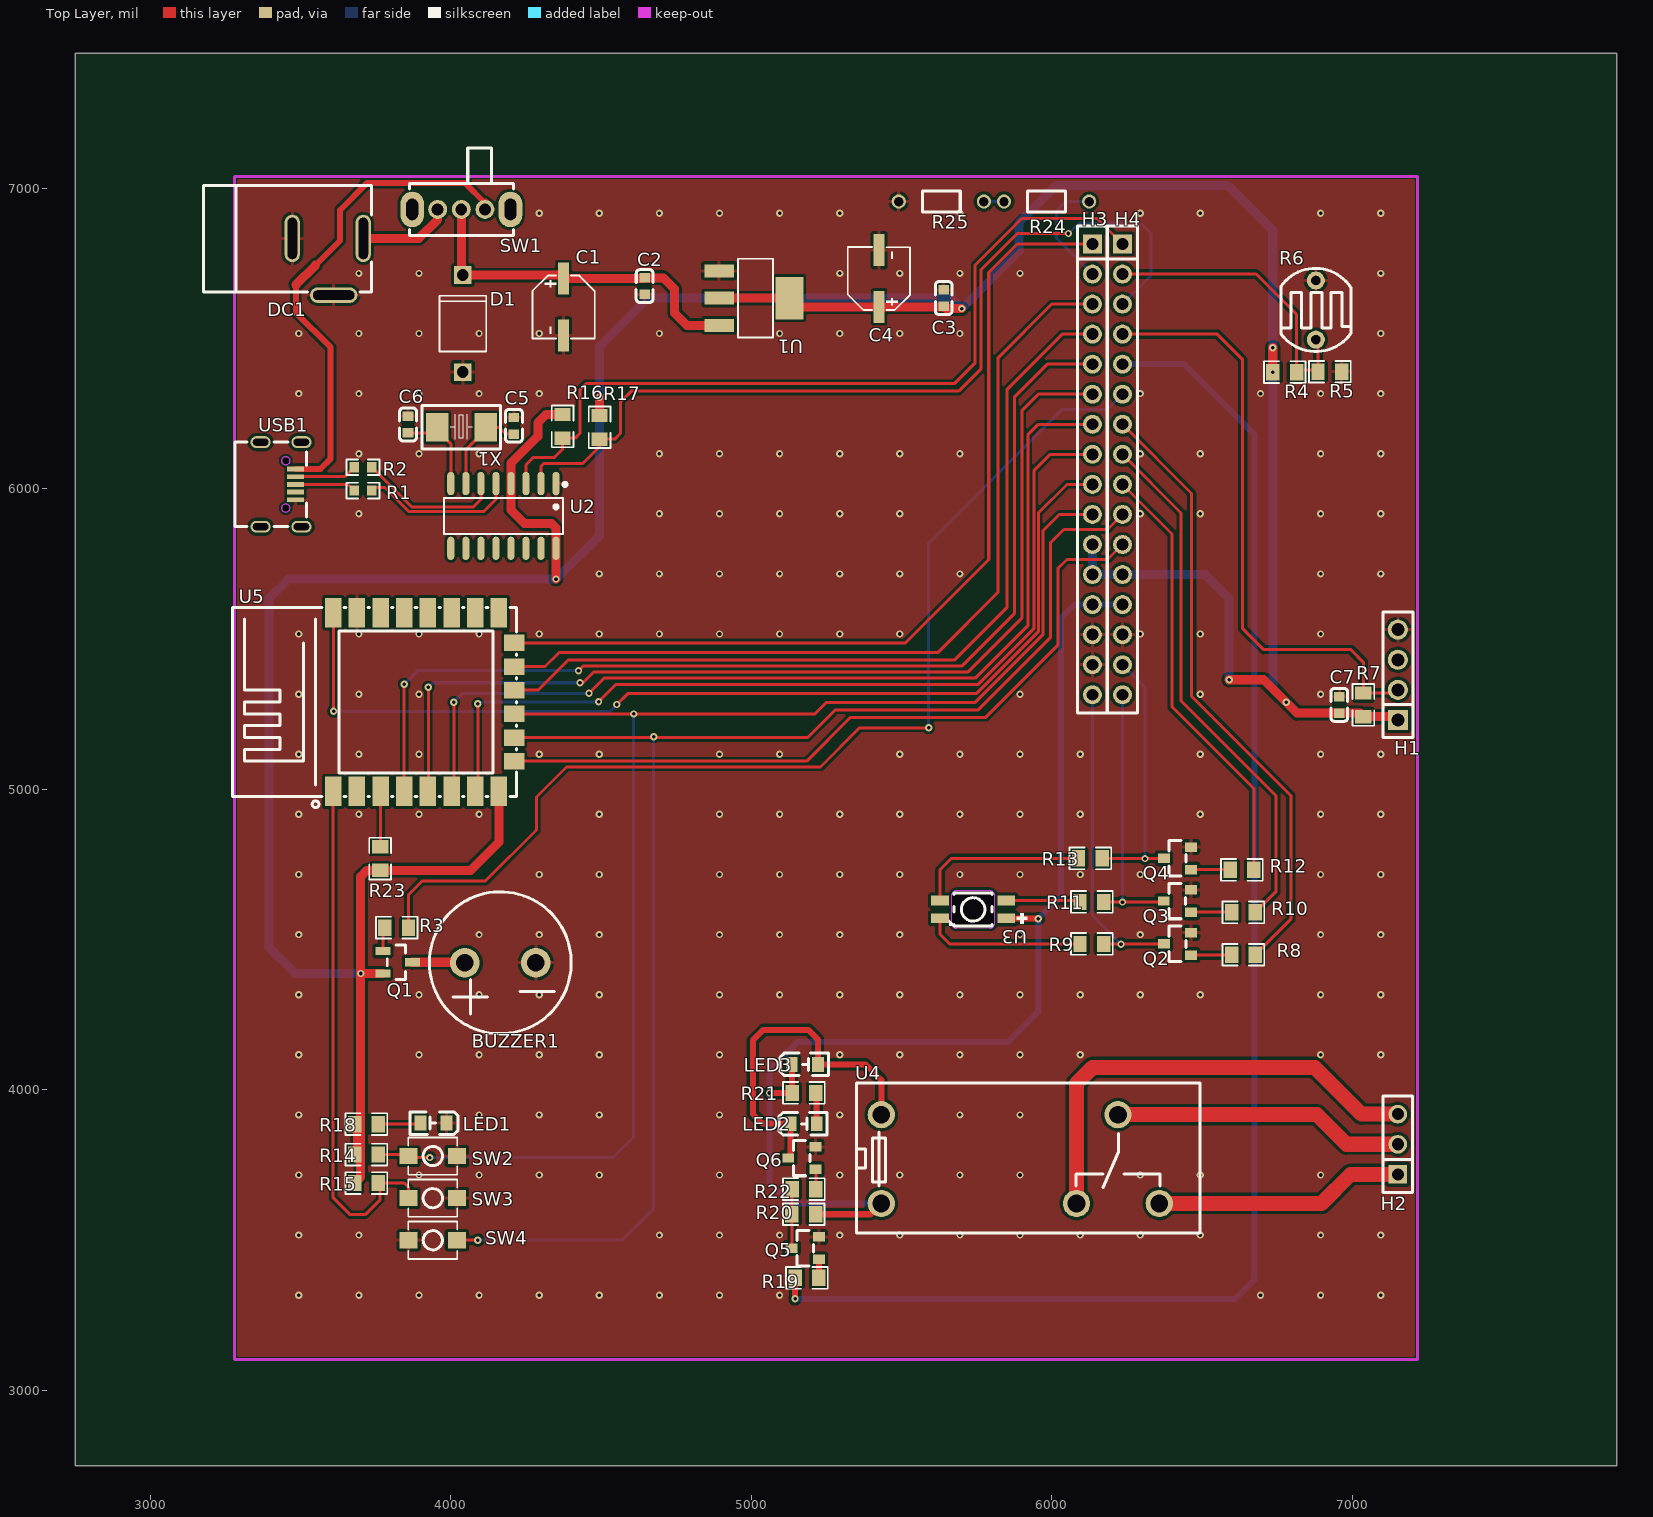
[diagram p0: Top Layer view]
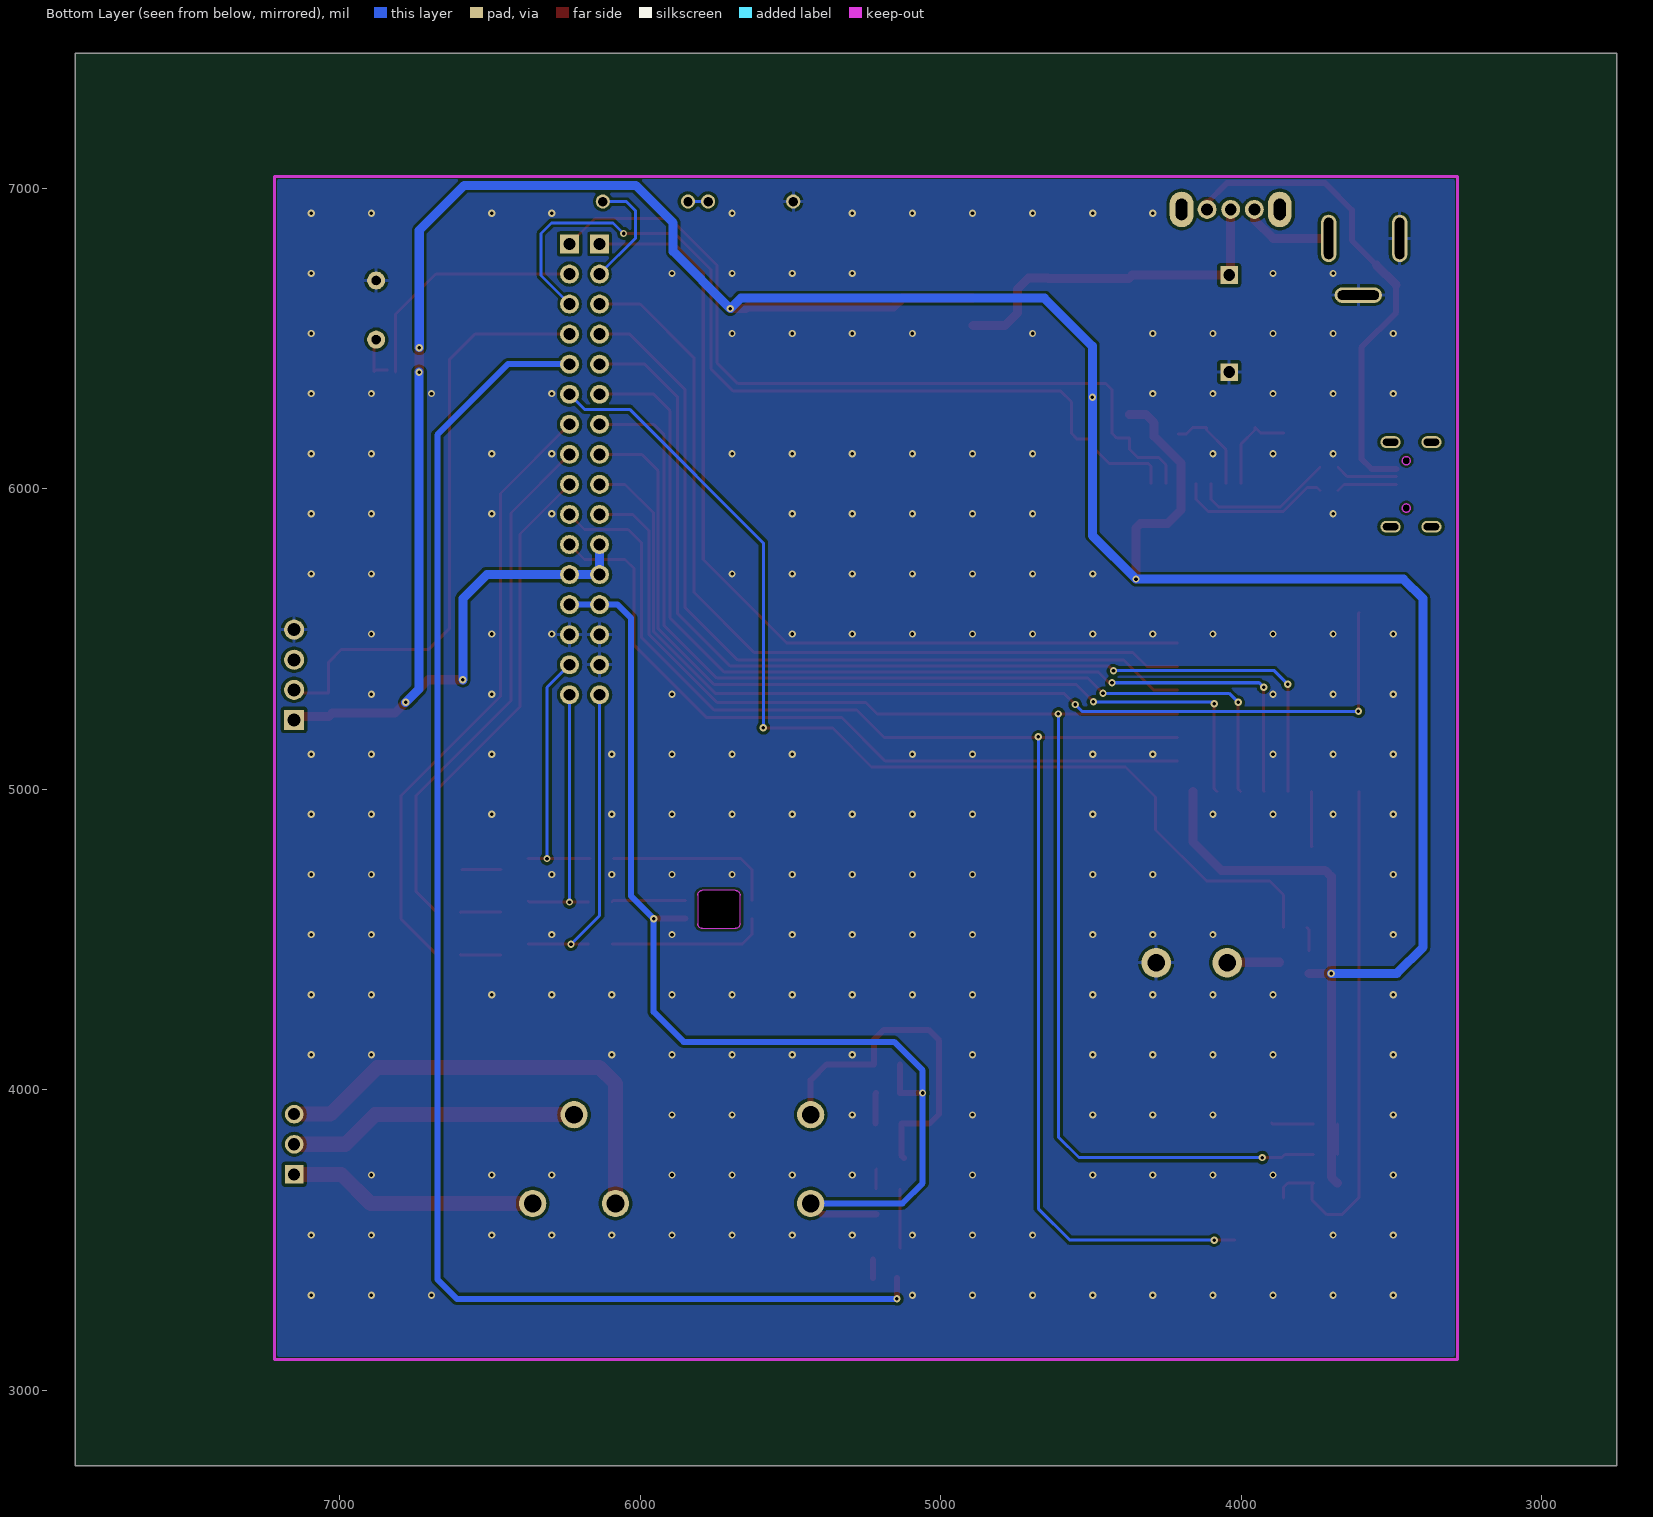
[diagram p1: Bottom Layer view, seen from below]
# Altium PCB MISC51905.pcbdoc
Units mil, origin at the board's own origin, x right, y up, seen from the top; angles counter-clockwise.
Board outline 5130 x 4700 mil, 2 copper layers (Top Layer, Bottom Layer), stack 62.206 mil thick; 59 components, 57 nets, 207 pads, 250 vias.

## Layer stack, top to bottom
Top Solder Mask Layer: solder mask 0.394, Dk 3.3
Top Layer: signal copper 1.379
Dielectric1: surface 59.449, FR4, Dk 4.5
Bottom Layer: signal copper 1.378
Bottom Solder Mask Layer: solder mask 0.394, Dk 3.3

## Board outline
7880,2750 2750,2750 2750,7450 7880,7450

## Design rules (kind name [scope] priority, off if disabled: settings)
BoardOutlineClearance copperThickness2oz_1 [All] p2 off: genericclearance=7.99 ignorepadtopadclearanceinfootprint=FALSE except(0: Arc-SplitContinuation Track-SplitContinuation SMDPad-SplitContinuation THPad-SplitContinuation Via-SplitContinuation Fill-SplitContinuation Region-SplitContinuation Poly-SplitContinuation Text-SplitContinuation Hole-SplitContinuation; 5.98: Arc-CutoutEdge SMDPad-CutoutEdge THPad-CutoutEdge Via-CutoutEdge Fill-CutoutEdge Region-CutoutEdge Text-CutoutEdge; 6.93: Hole-OutlineEdge Hole-CutoutEdge; 10: Poly-OutlineEdge Poly-CutoutEdge; 11.81: Arc-OutlineEdge Track-OutlineEdge SMDPad-OutlineEdge THPad-OutlineEdge Via-OutlineEdge Fill-OutlineEdge Region-OutlineEdge Text-OutlineEdge Track-CutoutEdge)
BoardOutlineClearance copperThickness1oz_1 [All] p4: genericclearance=4.02 ignorepadtopadclearanceinfootprint=FALSE except(0: Arc-SplitContinuation Track-SplitContinuation SMDPad-SplitContinuation THPad-SplitContinuation Via-SplitContinuation Fill-SplitContinuation Region-SplitContinuation Poly-SplitContinuation Text-SplitContinuation Hole-SplitContinuation; 6: SMDPad-CutoutEdge THPad-CutoutEdge Via-CutoutEdge Fill-CutoutEdge Region-CutoutEdge Text-CutoutEdge; 6.93: Hole-OutlineEdge Hole-CutoutEdge; 10: Poly-OutlineEdge Poly-CutoutEdge; 11.8: Arc-OutlineEdge Track-OutlineEdge SMDPad-OutlineEdge THPad-OutlineEdge Via-OutlineEdge Fill-OutlineEdge Region-OutlineEdge Text-OutlineEdge; 11.81: Arc-CutoutEdge Track-CutoutEdge)
Clearance copperThickness2oz [All] p1 off: gap=7.99 ignorepadtopadclearanceinfootprint=FALSE except(5.98: SMDPad-Track SMDPad-SMDPad THPad-Track SMDPad-THPad THPad-THPad Track-Via SMDPad-Via THPad-Via Via-Via Fill-Track Region-Track Fill-SMDPad Region-SMDPad Fill-THPad Region-THPad Fill-Via Region-Via Fill-Fill Fill-Region Region-Region Arc-Track Arc-SMDPad Arc-THPad Arc-Via Fill-Arc Region-Arc Arc-Arc Text-Track SMDPad-Text Text-THPad Text-Via Fill-Text Region-Text Arc-Text Text-Text; 6.93: Hole-Track Hole-SMDPad Hole-THPad Hole-Via Fill-Hole Region-Hole Hole-Arc Hole-Text; 10: Poly-Track Poly-SMDPad Poly-THPad Poly-Via Poly-Fill Poly-Region Poly-Poly Poly-Arc Poly-Text Poly-Hole)
Clearance copperThickness1oz [All] p3: gap=4.02 ignorepadtopadclearanceinfootprint=FALSE except(5.98: SMDPad-Track SMDPad-SMDPad THPad-Track SMDPad-THPad THPad-THPad Track-Via SMDPad-Via THPad-Via Via-Via Fill-Track Region-Track Fill-SMDPad Region-SMDPad Fill-THPad Region-THPad Fill-Via Region-Via Fill-Fill Fill-Region Region-Region; 6: Arc-Track Arc-SMDPad Arc-THPad Arc-Via Fill-Arc Region-Arc Arc-Arc Text-Track SMDPad-Text Text-THPad Text-Via Fill-Text Region-Text Arc-Text Text-Text; 6.93: Hole-Track Hole-SMDPad Hole-THPad Hole-Via Fill-Hole Region-Hole Hole-Arc Hole-Text; 10: Poly-Track Poly-SMDPad Poly-THPad Poly-Via Poly-Fill Poly-Region Poly-Poly Poly-Arc Poly-Text Poly-Hole)
DiffPairsRouting differentialPair [All] p1: maxlimit=6 minlimit=6 mostfreqgap=6 toplayer_minwidth=5 toplayer_prefwidth=10 toplayer_maxwidth=100 toplayer_mingap=6 toplayer_prefgap=6 toplayer_maxgap=6 bottomlayer_minwidth=5 bottomlayer_prefwidth=10 bottomlayer_maxwidth=100 bottomlayer_mingap=6 bottomlayer_prefgap=6 bottomlayer_maxgap=6 maxuncoupledlength=10
HoleToHoleClearance otherClearance [All] p1: gap=11.81 allowstackedmicrovias=TRUE
Length netLength [All] p1: minlimit=0 maxlimit=0
MatchedLengths netLengthTolerance [All] p1: tolerance=1000
PasteMaskExpansion pasteMaskExpansion [All] p1: expansion=0
PlaneConnect innerPlane [All] p1: planeconnectstyle=Relief reliefexpansion=20 reliefentries=4 reliefconductorwidth=10 reliefairgap=10
PolygonConnect copperRegion [(InNet('GND'))] p1: connectstyle=Relief reliefconductorwidth=10 reliefentries=4 polygonreliefangle="90 Angle" airgapwidth=10 via.connectstyle=Relief via.reliefconductorwidth=10 via.reliefentries=4 via.polygonreliefangle="90 Angle" via.airgapwidth=10
RoutingVias viaSize [All] p1: holewidth=12.01 width=24.02 viastyle="Through Hole" minholewidth=11.81 minwidth=19.68 maxholewidth=248.03 maxwidth=393.7
SolderMaskExpansion solderMaskExpansion [IsVia] p1: expansion=-1000 istentingtop=TRUE
SolderMaskExpansion solderMaskExpansion [All] p2: expansion=2 istentingtop=FALSE
Width copperThickness2oz_2 [All] p1 off: maxlimit=100 minlimit=8 preferedwidth=10
Width copperThickness1oz_2 [All] p2: maxlimit=100 minlimit=5 preferedwidth=10

## Components (designator, comment, footprint, x,y, rotation, side; value= is the part's Value field where it differs from the comment)
BUZZER1 "buzzer" BUZ-TH_BD12.0-P6.00-D0.9-RD 4164.88,4423.36 r180 top
C1 "10uF" C_Ele_SMD_5x5.4mm 4375,6605 r270 top
C2 "100nF" C0603 4645,6675 r90 top
C3 "100nF" C0603 5640,6635 r270 top
C4 "10uF" C_Ele_SMD_5x5.4mm 5425,6700 r90 top
C5 "22pF" C0603 4210,6210 r270 top
C6 "22pF" C0603 3857.75,6214.29 r270 top
C7 "100nF" C0603 6956.48,5281.48 r270 top
D1 "SMA_DIODE" SOD-57_BD3.8-L4.6-P9.00-D0.8-RD 4040,6550 r270 top
DC1 "" DC-2.0 3585.7,6844.2 r180 top
H1 "" HDR-TH_4P-P2.54-V-F 7151.48,5381.48 r90 top
H2 "" HDR-TH_3P-P2.54-V-F 7151.08,3819.36 r90 top
H3 "" HDR-TH_16P-P2.54-V-F 6135,6065 r270 top
H4 "" HDR-TH_16P-P2.54-V-F 6235,6065 r270 top
LED1 "" LED_0805 3940,3890 r180 top
LED2 "" LED_0805 5176.09,3887.47 r0 top
LED3 "" LED_0805 5180,4085 r0 top
Q1 "" S8550P_SOT 3825,4425 r180 top
Q2 "" S8050_SOT-23 6418.13,4485.78 r0 top
Q3 "" S8050_SOT-23 6417.7,4628.77 r0 top
Q4 "" S8050_SOT-23 6418.13,4770.78 r0 top
Q5 "" S8050_SOT-23 5179.42,3473.63 r0 top
Q6 "" S8050_SOT-23 5168.07,3773.63 r0 top
R1 "27R" R0603 3707.89,5994.43 r180 top
R2 "27R" R0603 3707.89,6072.13 r180 top
R3 "1K" R0805 3820,4540 r180 top
R4 "10K" R0805 6774.9,6388.36 r0 top
R5 "4.7K" R0805 6925,6390 r0 top
R6 "GL7528" RES-TH_L7.0-W5.9-P5.00-D0.5 6878.39,6595.1 r0 top
R7 "4.7K" R0805 7036.48,5281.48 r270 top
R8 "1.5K" R0805 6637.43,4450.05 r180 top
R9 "1K" R0805 6133.13,4485.78 r180 top
R10 "1.5K" R0805 6637.43,4591.12 r180 top
R11 "1K" R0805 6133.13,4625.78 r180 top
R12 "1.5K" R0805 6632.43,4732.47 r180 top
R13 "1K" R0805 6128.13,4770.78 r180 top
R14 "10K" R0805 3719.38,3785 r0 top
R15 "10K" R0805 3719.38,3690.3 r0 top
R16 "10K" R0805 4371.73,6208.26 r270 top
R17 "10K" R0805 4495,6205 r270 top
R18 "4.7K" R0805 3719.38,3886.21 r0 top
R19 "1.5K" R0805 5185,3375 r0 top
R20 "1.5K" R0805 5174.42,3586.47 r0 top
R21 "10K" R0805 5175,3990 r180 top
R22 "1.5K" R0805 5175,3670 r0 top
R23 "10K" R0805 3765,4770 r90 top
R24 "10K" Res_1/8W 5982.44,6953.68 r0 top
R25 "4.7K" Res_1/8W 5632.16,6953.68 r0 top
SW1 "" 拨动开关_侧 4035,6930 r180 top
SW2 "" Key_SMD_3x4x2 3940,3780 r0 top
SW3 "" Key_SMD_3x4x2 3940,3640 r0 top
SW4 "" Key_SMD_3x4x2 3940,3500 r180 top
U1 "AMS1117-3.3" SOT-223-3_L6.5-W3.4-P2.30-LS7.0-BR 5010,6635 r180 top
U2 "CH340G" SOIC-16_L9.9-W3.9-P1.27-LS6.0-BL 4175,5910 r180 top
U3 "6028-ZRGBF-SMD-H2" LED-SMD_4P-L3.2-W2.8_ZRGBF-SMD-H2 5738.13,4600.78 r180 top
U4 "SSKD6132" RELAY-TH_G2R-1 5895,3770 r0 top
U5 "ESP8266" WIFIM-SMD_ESP-12F-ESP8266MOD 3909.99,5290.81 r0 top
USB1 "" USB_Micro 3435,6015 r270 top
X1 "CRYSTAL" CRYSTAL-SMD_L5.0-W3.2 4035,6205 r180 top

## Footprints (in the part's own frame and the unit in brackets; to place one, negate y for a bottom-side part, rotate by r counter-clockwise, add the part's x,y. Pads: shape width x height; smd on the part's side, far side on the other; paste and mask are expansions set on the pad)
BUZ-TH_BD12.0-P6.00-D0.9-RD [mm]
  round 2.5 hole 1.5 paste+0 mask+0.05: 1(-3,0) 2(3,0)
  silkscreen extent -5.99,-5.99 5.99,5.99
C0603 [mm]
  rect 0.8x0.9 smd: 1(-0.7,0) 2(0.7,0)
  silkscreen extent -1.39,-0.71 1.39,0.71
C_Ele_SMD_5x5.4mm [mm]
  rect 2.7x0.91 smd paste+0 mask+0.051: 1(-2.4,0) 2(2.4,0)
  silkscreen extent -2.66,-2.62 2.66,2.65
CRYSTAL-SMD_L5.0-W3.2 [mm]
  rect 1.9x2.4 smd: 1(-2.05,0) 2(2.05,0)
  silkscreen extent -3.32,-1.85 3.33,1.85
DC-2.0 [mil]
  oval 157.5x51.2 hole 31.5 slot 137.8 at 0 deg paste+0 mask+2: 2(-24.7,199.5)
  oval 51.2x157.5 hole 31.5 slot 137.8 at 90 deg paste+0 mask+2: 3(113.1,10.5) 4(-123.1,10.5)
  silkscreen extent -151,-165 408,190
HDR-TH_3P-P2.54-V-F [mil]
  rect 62x62 hole 40.16: 1(-100,0)
  round 62 hole 40.16: 2(0,0) 3(100,0)
  silkscreen extent -160,-49 160,49
HDR-TH_4P-P2.54-V-F [mm]
  rect 1.7x1.7 hole 1.1: 1(-3.81,0)
  round 1.7 hole 1.1: 2(-1.27,0) 3(1.27,0) 4(3.81,0)
  silkscreen extent -5.29,-1.27 5.29,1.27
HDR-TH_16P-P2.54-V-F [mm]
  rect 1.6x1.6 hole 1: 1(-19.05,0)
  round 1.6 hole 1: 2(-16.51,0) 3(-13.97,0) 4(-11.43,0) 5(-8.89,0) 6(-6.35,0) 7(-3.81,0) 8(-1.27,0) 9(1.27,0) 10(3.81,0) 11(6.35,0) 12(8.89,0) 13(11.43,0) 14(13.97,0) 15(16.51,0) 16(19.05,0)
  silkscreen extent -20.57,-1.25 20.57,1.25
Key_SMD_3x4x2 [mm]
  rect 1.53x1.36 smd paste+0 mask+0.051: 1(-2.035,0) 2(2.035,0)
  silkscreen extent -2.08,-1.58 2.08,1.58
LED-SMD_4P-L3.2-W2.8_ZRGBF-SMD-H2 [mm]
  rect 1.5x0.82 smd: 1(2.8,0.75) 2(-2.8,0.75) 3(2.8,-0.75) 4(-2.8,-0.75)
  Board Outline Layer lines w0.003: 1.8,1.2 ccw(c1.4,1.2) 1.4,1.6 -1.4,1.6 ccw(c-1.4,1.2) -1.8,1.2 -1.8,-1.2 ccw(c-1.4,-1.2) -1.406,-1.6 ccw(c-1.413,-1.2) -1.4,-1.6 1.4,-1.6 ccw(c1.4,-1.2) 1.8,-1.2 1.8,1.2
  Board Outline Layer region: 1.8,-1.2 1.79,-1.289 1.76,-1.374 1.713,-1.45 1.649,-1.513 1.574,-1.561 1.489,-1.59 1.4,-1.6 1.4,-1.6 -1.4,-1.6 -1.403,-1.6 -1.406,-1.6 -1.494,-1.589 -1.578,-1.559 -1.652,-1.511 -1.714,-1.448 -1.761,-1.372 -1.79,-1.288 -1.8,-1.2 -1.8,-1.2 -1.8,-1.2 -1.8,1.2 -1.79,1.289 -1.76,1.374 -1.713,1.449 -1.649,1.513 -1.574,1.56 -1.489,1.59 -1.4,1.6 1.4,1.6 1.4,1.6 1.489,1.59 1.574,1.561 1.649,1.513 1.713,1.45 1.76,1.374 1.79,1.289 1.8,1.2 1.8,-1.2
  Board Outline Layer region: 1.8,-1.2 1.79,-1.289 1.76,-1.374 1.713,-1.45 1.649,-1.513 1.574,-1.561 1.489,-1.59 1.4,-1.6 1.4,-1.6 -1.4,-1.6 -1.403,-1.6 -1.406,-1.6 -1.494,-1.589 -1.578,-1.559 -1.652,-1.511 -1.714,-1.448 -1.761,-1.372 -1.79,-1.288 -1.8,-1.2 -1.8,-1.2 -1.8,-1.2 -1.8,1.2 -1.79,1.289 -1.76,1.374 -1.713,1.449 -1.649,1.513 -1.574,1.56 -1.489,1.59 -1.4,1.6 1.4,1.6 1.4,1.6 1.489,1.59 1.574,1.561 1.649,1.513 1.713,1.45 1.76,1.374 1.79,1.289 1.8,1.2 1.8,-1.2
  Multi-Layer board cut-out: 1.8,-1.2 1.79,-1.289 1.76,-1.374 1.713,-1.45 1.649,-1.513 1.574,-1.561 1.489,-1.59 1.4,-1.6 1.4,-1.6 -1.4,-1.6 -1.403,-1.6 -1.406,-1.6 -1.494,-1.589 -1.578,-1.559 -1.652,-1.511 -1.714,-1.448 -1.761,-1.372 -1.79,-1.288 -1.8,-1.2 -1.8,-1.2 -1.8,-1.2 -1.8,1.2 -1.79,1.289 -1.76,1.374 -1.713,1.449 -1.649,1.513 -1.574,1.56 -1.489,1.59 -1.4,1.6 1.4,1.6 1.4,1.6 1.489,1.59 1.574,1.561 1.649,1.513 1.713,1.45 1.76,1.374 1.79,1.289 1.8,1.2 1.8,-1.2
  silkscreen extent -4.57,-1.4 2.03,1.4
LED_0805 [mm]
  rect 1x1.25 smd paste+0 mask+0.051: 1(-1.15,0.005) 2(1.05,0.005)
  silkscreen extent -2.15,-0.94 1.93,0.97
R0603 [mil]
  rect 31.75x34.02 smd paste-3937.01 mask+2: 1(-29.66,0) 2(29.66,0)
  silkscreen extent -55,-26 55,26
R0805 [mm]
  rect 1.133x1.377 smd paste-100 mask+0.051: 1(-1,0) 2(1,0)
  silkscreen extent -1.76,-0.92 1.76,0.92
RELAY-TH_G2R-1 [mm]
  round 2.3 hole 1.5: 1(-11.75,-3.75) 2(4.75,-3.75) 3(11.75,-3.75) 4(8.25,3.75) 5(-11.75,3.75)
  silkscreen extent -13.83,-6.26 15.17,6.44
RES-TH_L7.0-W5.9-P5.00-D0.5 [mil]
  round 60 hole 30 slot 30.2 at 90 deg: 1(0,-98.42) 2(0,98.43)
  silkscreen extent -116,-138 116,139
Res_1/8W [mil]
  round 47.2 hole 31.5 paste+0 mask+2: 1(-141.7,2.48) 2(141.7,2.48)
  silkscreen extent -63,-33 63,38
S8050_SOT-23 [mm]
  rect 1x0.8 smd paste+0 mask+0.051: 1(1.15,-0.95) 2(1.15,0.95) 3(-1.15,0)
  silkscreen extent -0.7,-1.5 0.7,1.5
S8550P_SOT [mil]
  rect 49.2x27.6 smd paste+0 mask+2: 1(50.84,-37.4) 2(50.84,37.4) 3(-47.56,0)
  silkscreen extent -24,-58 37,58
SOD-57_BD3.8-L4.6-P9.00-D0.8-RD [mm]
  rect 1.5x1.5 hole 1: 1(-4.1,0) 2(4.1,0)
  silkscreen extent -2.36,-1.98 2.36,1.98
SOIC-16_L9.9-W3.9-P1.27-LS6.0-BL [mil]
  oval 23.7x77.6 smd: 1(-175,-107.7) 2(-125,-107.7) 3(-75,-107.7) 4(-25,-107.7) 5(25,-107.7) 6(75,-107.7) 7(125,-107.7) 8(175,-107.7) 9(175,107.7) 10(125,107.7) 11(75,107.7) 12(25,107.7) 13(-25,107.7) 14(-75,107.7) 15(-125,107.7) 16(-175,107.7)
  silkscreen extent -211,-111 198,60
SOT-223-3_L6.5-W3.4-P2.30-LS7.0-BR [mm]
  rect 2.5x1.1 smd: 1(2.97,-2.3) 2(2.97,0) 3(2.97,2.3)
  rect 2.34x3.6 smd: 4(-2.97,0)
  silkscreen extent -1.57,-3.33 1.37,3.33
USB_Micro [mm]
  rect 0.4x1.4 smd paste-100 mask+0.05: 1(-1.3,1.225) 2(-0.65,1.225) 3(0,1.225) 4(0.65,1.225) 5(1.3,1.225)
  oval 1x1.7 hole 0.6 slot 1.3 at 90 deg paste+0 mask+0.05: 6(-3.575,-1.725) 6(-3.575,1.725) 6(3.575,-1.725) 6(3.575,1.725)
  Board Outline Layer circle w0.003: c-2,0.4 r0.35
  Board Outline Layer circle w0.003: c2,0.4 r0.35
  Board Outline Layer region: -2,0.75 -1.848,0.715 -1.726,0.618 -1.659,0.478 -1.659,0.322 -1.726,0.182 -1.848,0.085 -2,0.05 -2,0.05 -2.152,0.085 -2.274,0.182 -2.341,0.322 -2.341,0.478 -2.274,0.618 -2.152,0.715 -2,0.75
  Board Outline Layer region: -2,0.75 -1.922,0.741 -1.848,0.715 -1.782,0.674 -1.726,0.618 -1.685,0.552 -1.659,0.478 -1.65,0.4 -1.659,0.322 -1.685,0.248 -1.726,0.182 -1.782,0.126 -1.848,0.085 -1.922,0.059 -2,0.05 -2.078,0.059 -2.152,0.085 -2.218,0.126 -2.274,0.182 -2.315,0.248 -2.341,0.322 -2.35,0.4 -2.341,0.478 -2.315,0.552 -2.274,0.618 -2.218,0.674 -2.152,0.715 -2.078,0.741
  Board Outline Layer region: 2,0.75 2.152,0.715 2.274,0.618 2.341,0.478 2.341,0.322 2.274,0.182 2.152,0.085 2,0.05 2,0.05 1.848,0.085 1.726,0.182 1.659,0.322 1.659,0.478 1.726,0.618 1.848,0.715 2,0.75
  Board Outline Layer region: 2,0.75 2.078,0.741 2.152,0.715 2.218,0.674 2.274,0.618 2.315,0.552 2.341,0.478 2.35,0.4 2.341,0.322 2.315,0.248 2.274,0.182 2.218,0.126 2.152,0.085 2.078,0.059 2,0.05 1.922,0.059 1.848,0.085 1.782,0.126 1.726,0.182 1.685,0.248 1.659,0.322 1.65,0.4 1.659,0.478 1.685,0.552 1.726,0.618 1.782,0.674 1.848,0.715 1.922,0.741
  Multi-Layer board cut-out: -2,0.75 -1.848,0.715 -1.726,0.618 -1.659,0.478 -1.659,0.322 -1.726,0.182 -1.848,0.085 -2,0.05 -2,0.05 -2.152,0.085 -2.274,0.182 -2.341,0.322 -2.341,0.478 -2.274,0.618 -2.152,0.715 -2,0.75
  Multi-Layer board cut-out: 2,0.75 2.152,0.715 2.274,0.618 2.341,0.478 2.341,0.322 2.274,0.182 2.152,0.085 2,0.05 2,0.05 1.848,0.085 1.726,0.182 1.659,0.322 1.659,0.478 1.726,0.618 1.848,0.715 2,0.75
  silkscreen extent -3.57,-3.87 3.57,2.14
WIFIM-SMD_ESP-12F-ESP8266MOD [mm]
  rect 1.4x2.5 smd: 1(-7.651,-7.551) 2(-5.651,-7.551) 3(-3.651,-7.551) 4(-1.651,-7.551) 5(0.349,-7.551) 6(2.349,-7.551) 7(4.349,-7.551) 8(6.349,-7.551) 9(6.349,7.549) 10(4.349,7.55) 11(2.349,7.551) 12(0.349,7.551) 13(-1.651,7.55) 14(-3.651,7.551) 15(-5.651,7.55) 16(-7.651,7.551)
  rect 1.7x1.4 smd: 17(7.651,-5) 18(7.649,-3.002) 19(7.65,-1.003) 20(7.65,0.997) 21(7.65,2.997) 22(7.65,4.997)
  silkscreen extent -16.15,-8.92 7.85,8
拨动开关_侧 [mil]
  round 63 hole 39.4 paste+0 mask+2: 1(-78.7,0) 2(0,0) 3(78.7,0)
  oval 78.7x118.1 hole 39.4 slot 70.9 at 90 deg paste+0 mask+2: 4(163.4,0) 5(-163.4,0)
  silkscreen extent -173,-205 173,87

## Via types
v1: diameter 24.02, hole 12, Top Layer to Bottom Layer, 250 vias

## Nets (pads, with @x,y where several pads share a name; then routed paths per layer and width w, separated by ;. In a path a pad name is that pad's centre, name@x,y a point inside that pad or via, vN(x,y) a via of type N, cw(c..) or ccw(c..) an arc to the next point about the centre after c; other vN are vias at no path point)
5V: H3.13 H4.13 LED3.1 R20.2 R21.2 U3.2 U4.1 | length 3827.7
  Top Layer w20: v1(5060,3990) R21.2 5134.72,3990.91 LED3.1 ; R20.2 5396.52,3586.47 U4.1 ; U3.2 5849.63,4570 v1(5955,4570)
  Bottom Layer w20: U4.1 5127.65,3622.35 5060,3690 v1(5060,3990) 5060,4065 5155,4160 5855,4160 5955,4260 v1(5955,4570) 6030,4645 6030,5570 6075,5615 H3.13 H4.13
8266_RESET: R15.2 SW3.1 U5.1 | length 1752.9
  Top Layer w10: U5.1 3608.79,3641.21 3665,3585 3715,3585 3765,3635 3765,3684.05 R15.2 3844.7,3690.3 3859.88,3675.12 SW3.1
$1N2: DC1.4 SW1.3 | length 307.1
  Top Layer w30: DC1.4 3893.7,6833.7 3956.3,6896.3 SW1.3
$1N13: C5.2 U2.7 X1.1 | length 318.1
  Top Layer w10: U2.7 4050,6130 4115.71,6195.71 X1.1 4160,6205 4182.56,6182.44 C5.2
$1N14: C6.2 U2.8 X1.2 | length 310.3
  Top Layer w10: C6.2 3936.02,6186.73 X1.2 3954.29,6195.71 4000,6150 U2.8
$1N19: R1.2 USB1.3 | length 203.5
  Top Layer w10: USB1.3 3657.67,6015 R1.2
$1N20: R2.2 USB1.2 | length 208.1
  Top Layer w10: USB1.2 3646.69,6040.59 R2.2
$1N25: Q1.1 R3.2 | length 80.3
  Top Layer w10: Q1.1 3774.16,4533.53 R3.2
$1N27: BUZZER1.2 Q1.3 | length 174.9
  Top Layer w30: Q1.3 4045.13,4425 BUZZER1.2
$1N37: Q2.1 R8.2 | length 135.3
  Top Layer w10: Q2.1 6596.39,4448.38 R8.2
$1N41: R9.2 U3.1 | length 532.4
  Top Layer w10: U3.1 5627.89,4518.11 5660.22,4485.78 R9.2
$1N44: R11.2 U3.4 | length 247.3
  Top Layer w10: U3.4 6089.23,4630.31 R11.2
$1N46: Q3.1 R10.2 | length 135.2
  Top Layer w10: Q3.1 6597.81,4591.37 R10.2
$1N48: R13.2 U3.3 | length 579.1
  Top Layer w10: U3.3 5627.89,4732.89 5665.78,4770.78 R13.2
$1N50: Q4.1 R12.2 | length 130
  Top Layer w10: Q4.1 6592.15,4733.38 R12.2
$1N61: LED1.2 R18.2 | length 141.4
  Top Layer w10: R18.2 3895.07,3886.21 LED1.2
$1N66: Q5.1 R19.2 | length 61.4
  Top Layer w20: R19.2 5224.7,3375.33 Q5.1
$1N68: Q5.3 R20.1 R22.1 | length 197
  Top Layer w10: Q5.3 5135.63,3475.11 R22.1
$1N70: LED2.2 R21.1 | length 103.6
  Top Layer w20: R21.1 5217.43,3986.94 LED2.2
$1N71: LED2.1 LED3.2 Q6.3 U4.5 | length 1176.6
  Top Layer w20: Q6.3 5130.81,3781.64 LED2.1 5037.33,3887.67 5005,3920 5005,4165 5040,4200 5190,4200 5221.34,4168.66 LED3.2 5379.8,4085.2 5432.4,4032.6 U4.5
$1N73: Q6.1 R22.2 | length 66.6
  Top Layer w10: Q6.1 5214.37,3735.21 R22.2
$1N74: H2.1 U4.3 | length 833.7
  Top Layer w50: U4.3 6897.35,3622.35 6994.36,3719.36 H2.1
$1N75: H2.2 U4.4 | length 972
  Top Layer w50: U4.4 6882.35,3917.65 6980.64,3819.36 H2.2
$1N76: H2.3 U4.2 | length 1555.2
  Top Layer w50: U4.2 6082,4022 6135,4075 6875,4075 7030.64,3919.36 H2.3
$1N152: H3.2 R24.2 | length 381.8
  Bottom Layer w10: R24.2 6046.16,6956.16 6015,6925 6015,6835 H3.2
+5V: C1.1 C2.2 D1.1 SW1.2 U1.3 | length 1192.3
  Top Layer w30: SW1.2 4035,6716.42 D1.1 4363.07,6711.42 C1.1 4641.93,6699.49 C2.2 4707.44,6702.56 4745,6665 4745,6585 4785.55,6544.45 U1.3
ADC: H4.2 R4.2 R5.1 R6.1 | length 984.6
  Top Layer w10: H4.2 6680,6715 6814.27,6580.73 R4.2 ; 6840,6395 6880.63,6395 R5.1 6885.63,6489.44 R6.1
B: H4.15 Q4.3 R13.1 | length 881.4
  Top Layer w10: R13.1 Q4.3
  Bottom Layer w10: H4.15 6310,5340 v1(6310,4770)
CH_PD: R23.2 U5.3 | length 184.7
  Top Layer w10: R23.2 3766.27,4810.64 U5.3
D+: R1.1 U2.5 | length 519.2
  Top Layer w10: R1.1 3748.12,6005 3780,6005 3860,5925 4110,5925 4150,5965 U2.5
D-: R2.1 U2.6 | length 480.2
  Top Layer w10: R2.1 3869.69,5940 4075,5940 4100,5965 U2.6
ESP8266-ADC: R24.1 R25.2 | length 66.9
  Bottom Layer w10: R25.2 R24.1
ESP8266_ADC: U5.2
ESP8266_IO0: H4.10 SW4.1 U5.18 | length 4784.3
  Top Layer w10: SW4.1 v1(4090,3500) ; U5.18 5187.62,5172.62 5280,5265 5755,5265 5995,5505 5995,5820 6040,5865 6185,5865 H4.10
  Bottom Layer w10: v1(4090,3500) 4570,3500 4675,3605 v1(4675,5175)
ESP8266_IO2: H4.11 U5.17 | length 2471.8
  Top Layer w10: U5.17 5183.96,5093.96 5330,5240 5780,5240 6020,5480 6020,5735 6050,5765 6185,5765 H4.11
ESP8266_IO4: H3.10 R14.2 SW2.1 U5.19 | length 4690.9
  Top Layer w10: R14.2 3854.88,3785 SW2.1 3864.88,3775 v1(3930,3775) ; U5.19 v1(4608.39,5251.31) 5211.31,5251.31 5250,5290 5745,5290 5970,5515 5970,5860 6025,5915 H3.10
  Bottom Layer w10: v1(3930,3775) 4540,3775 4608.39,3843.39 v1(4608.39,5251.31)
ESP8266_IO5: H3.4 U5.20 | length 2839.3
  Top Layer w10: U5.20 4290.08,5330.08 4390,5430 5675,5430 5850,5605 5850,6330 6035,6515 H3.4
ESP8266_IO12: H3.7 U5.6 | length 3179.7
  Top Layer w10: U5.6 4010,5001.03 v1(4010,5290) ; v1(4460,5320) 4510,5370 5745,5370 5920,5545 5920,6180 5955,6215 H3.7
  Bottom Layer w10: v1(4010,5290) 4040,5320 v1(4460,5320)
ESP8266_IO13: H3.8 U5.7 | length 2991.5
  Top Layer w10: U5.7 4090,5002.29 v1(4090,5285) ; v1(4491.66,5291.66) 4550,5350 5755,5350 5940,5535 5940,6060 5995,6115 H3.8
  Bottom Layer w10: v1(4090,5285) 4096.66,5291.66 v1(4491.66,5291.66)
ESP8266_IO14: H3.6 U5.5 | length 3365.1
  Top Layer w10: U5.5 3925,4994.77 v1(3925,5340) ; v1(4430,5355) 4440,5355 4475,5390 5720,5390 5900,5570 5900,6260 5955,6315 H3.6
  Bottom Layer w10: v1(3925,5340) 3940,5355 v1(4430,5355)
ESP8266_IO15: H3.9 U5.16 | length 3397.7
  Top Layer w10: U5.16 3610,5586.87 v1(3610,5260) ; v1(4552.5,5282.5) 4590,5320 5750,5320 5955,5525 5955,5920 6050,6015 H3.9
  Bottom Layer w10: v1(3610,5260) 4530,5260 v1(4552.5,5282.5)
ESP8266_IO16: H3.5 U5.4 | length 3509.4
  Top Layer w10: U5.4 v1(3845,5350) ; v1(4425,5395) 4440,5410 5700,5410 5875,5585 5875,6305 5985,6415 H3.5
  Bottom Layer w10: v1(3845,5350) 3890,5395 v1(4425,5395)
ESP8266_RX: H3.3 U5.21 | length 2880.4
  Top Layer w10: U5.21 4313.79,5408.79 4360,5455 5620,5455 5820,5655 5820,6435 6000,6615 H3.3
ESP8266_TX: H3.1 U5.22 | length 3033.1
  Top Layer w10: U5.22 5512.53,5487.53 5790,5765 5790,6720 5885,6815 H3.1
G: H4.16 Q3.3 R11.1 | length 891.2
  Top Layer w10: R11.1 6369.43,4625.78 Q3.3
  Bottom Layer w10: v1(6235,4625) H4.16
GND: BUZZER1.1 C1.2 C2.1 C3.1 C4.2 C5.1 C6.1 C7.1 D1.2 DC1.2 DC1.3 H1.4 H3.14 H3.15 H4.14 LED1.1 Q2.2 Q3.2 Q4.2 Q5.2 Q6.2 R5.2 R6.2 R25.1 SW2.2 SW3.2 SW4.2 U1.1 U2.1 U5.15 USB1.5
  other v1: 3494.1,3317.09 3694.1,3317.09 3894.1,3317.09 4094.1,3317.09 4294.1,3317.09 4494.1,3317.09 4694.1,3317.09 4894.1,3317.09 5094.1,3317.09 6694.1,3317.09 6894.1,3317.09 7094.1,3317.09 3494.1,3517.09 3694.1,3517.09 4694.1,3517.09 4894.1,3517.09 5094.1,3517.09 5294.1,3517.09 5494.1,3517.09 5694.1,3517.09 5894.1,3517.09 6094.1,3517.09 6294.1,3517.09 6494.1,3517.09 6894.1,3517.09 7094.1,3517.09 3494.1,3717.09 3894.1,3717.09 4094.1,3717.09 4294.1,3717.09 4494.1,3717.09 4894.1,3717.09 5294.1,3717.09 5494.1,3717.09 5694.1,3717.09 5894.1,3717.09 6294.1,3717.09 6494.1,3717.09 6894.1,3717.09 3494.1,3917.09 4094.1,3917.09 4294.1,3917.09 4494.1,3917.09 4894.1,3917.09 5294.1,3917.09 5694.1,3917.09 5894.1,3917.09 3494.1,4117.09 3894.1,4117.09 4094.1,4117.09 4294.1,4117.09 4494.1,4117.09 4894.1,4117.09 5294.1,4117.09 5494.1,4117.09 5694.1,4117.09 5894.1,4117.09 6094.1,4117.09 6894.1,4117.09 7094.1,4117.09 3494.1,4317.09 3894.1,4317.09 4094.1,4317.09 4294.1,4317.09 4494.1,4317.09 4894.1,4317.09 5094.1,4317.09 5294.1,4317.09 5494.1,4317.09 5694.1,4317.09 5894.1,4317.09 6094.1,4317.09 6294.1,4317.09 6494.1,4317.09 6894.1,4317.09 7094.1,4317.09 3494.1,4517.09 4094.1,4517.09 4294.1,4517.09 4494.1,4517.09 4894.1,4517.09 5094.1,4517.09 5294.1,4517.09 5494.1,4517.09 5894.1,4517.09 6294.1,4517.09 6894.1,4517.09 7094.1,4517.09 3494.1,4717.09 4294.1,4717.09 4494.1,4717.09 4894.1,4717.09 5094.1,4717.09 5294.1,4717.09 5494.1,4717.09 5694.1,4717.09 5894.1,4717.09 6094.1,4717.09 6294.1,4717.09 6894.1,4717.09 7094.1,4717.09 3494.1,4917.09 3694.1,4917.09 3894.1,4917.09 4094.1,4917.09 4494.1,4917.09 4894.1,4917.09 5094.1,4917.09 5294.1,4917.09 5494.1,4917.09 5694.1,4917.09 5894.1,4917.09 6094.1,4917.09 6494.1,4917.09 6894.1,4917.09 7094.1,4917.09 3494.1,5117.09 3694.1,5117.09 3894.1,5117.09 4294.1,5117.09 4494.1,5117.09 4894.1,5117.09 5094.1,5117.09 5494.1,5117.09 5694.1,5117.09 5894.1,5117.09 6094.1,5117.09 6494.1,5117.09 6894.1,5117.09 7094.1,5117.09 3494.1,5317.09 3694.1,5317.09 3894.1,5317.09 5894.1,5317.09 6494.1,5317.09 6894.1,5317.09 3494.1,5517.09 3694.1,5517.09 3894.1,5517.09 4094.1,5517.09 4294.1,5517.09 4494.1,5517.09 4694.1,5517.09 4894.1,5517.09 5094.1,5517.09 5294.1,5517.09 5494.1,5517.09 6294.1,5517.09 6494.1,5517.09 6894.1,5517.09 4494.1,5717.09 4694.1,5717.09 4894.1,5717.09 5094.1,5717.09 5294.1,5717.09 5494.1,5717.09 5694.1,5717.09 6894.1,5717.09 7094.1,5717.09 3694.1,5917.09 4694.1,5917.09 4894.1,5917.09 5094.1,5917.09 5294.1,5917.09 5494.1,5917.09 6294.1,5917.09 6494.1,5917.09 6894.1,5917.09 7094.1,5917.09 3694.1,6117.09 3894.1,6117.09 4094.1,6117.09 4694.1,6117.09 4894.1,6117.09 5094.1,6117.09 5294.1,6117.09 5494.1,6117.09 5694.1,6117.09 6294.1,6117.09 6494.1,6117.09 6894.1,6117.09 7094.1,6117.09 3494.1,6317.09 3694.1,6317.09 3894.1,6317.09 4094.1,6317.09 4294.1,6317.09 6294.1,6317.09 6694.1,6317.09 6894.1,6317.09 7094.1,6317.09 3494.1,6517.09 3694.1,6517.09 3894.1,6517.09 4094.1,6517.09 4294.1,6517.09 4694.1,6517.09 5094.1,6517.09 5294.1,6517.09 5494.1,6517.09 5694.1,6517.09 7094.1,6517.09 3694.1,6717.09 3894.1,6717.09 5294.1,6717.09 5494.1,6717.09 5694.1,6717.09 5894.1,6717.09 7094.1,6717.09 4294.1,6917.09 4494.1,6917.09 4694.1,6917.09 4894.1,6917.09 5094.1,6917.09 5294.1,6917.09 5694.1,6917.09 6294.1,6917.09 6494.1,6917.09 6894.1,6917.09 7094.1,6917.09
GPIO05: H1.2 H4.4 R7.1 | length 1999.9
  Top Layer w10: H4.4 6550,6515 6635,6430 6635,5535 6705,5465 6995,5465 7036.48,5423.52 R7.1 7140.85,5320.85 H1.2
GPIO12: H4.7 R8.1 | length 2045.9
  Top Layer w10: H4.7 6465,5985 6465,5310 6795,4980 6795,4568.25 R8.1
GPIO13: H4.8 R10.1 | length 1763.4
  Top Layer w10: H4.8 6430,5920 6430,5295 6745,4980 6745,4659.32 R10.1
GPIO14: H4.6 R3.1 | length 3599.6
  Top Layer w10: R3.1 3859.37,4649.37 3905,4695 4115,4695 4285,4865 4285,4975 4385,5075 5230,5075 5360,5205 v1(5590,5205)
  Bottom Layer w10: v1(5590,5205) 5590,5820 6035,6265 6185,6265 H4.6
GPIO15: H4.9 R12.1 | length 1463.5
  Top Layer w10: H4.9 6400,5850 6400,5275 6671.8,5003.2 R12.1
GPIO16: H4.5 R19.1 | length 4973.6
  Top Layer w20: v1(5145.63,3305) R19.1
  Bottom Layer w20: v1(5145.63,3305) 6610,3305 6675,3370 6675,6180 6440,6415 H4.5
R: H3.16 Q2.3 R9.1 | length 1069.7
  Top Layer w10: R9.1 Q2.3
  Bottom Layer w10: H3.16 6135,4580 v1(6230,4485)
VBUS: SW1.1 USB1.1 | length 1636.2
  Top Layer w20: USB1.1 3566.18,6066.18 3600,6100 3600,6470.89 3484.33,6586.56 3484.33,6679.33 ; 3550,6745 3631.62,6826.62 3631.62,6928.07 3721.75,7018.2 4046.8,7018.2 SW1.1@4113.7,6951.3
  Top Layer w30: 3484.33,6679.33 3550,6745 ; SW1.1 SW1.1@4113.7,6951.3
WIFI_3V3: C3.2 C4.1 C7.2 H1.1 H3.11 H3.12 H4.12 Q1.2 R4.1 R7.2 R14.1 R15.1 R16.1 R17.1 R18.1 R23.1 U1.2 U1.4 U2.4 U2.16 U5.8 | length 12518.6
  Top Layer w10: R14.1 R18.1
  Top Layer w30: R15.1 3700,3710.29 v1(3700,4387.6) ; Q1.2 v1(3700,4387.6) ; U5.8 4159.97,4824.97 4065.63,4730.63 R23.1 3720.63,4730.63 3700,4710 v1(3700,4387.6) ; v1(4350,5700) U2.16 4350,5870 4335,5885 4245,5885 4200,5930 U2.4 4200,6085 4290,6175 4290,6220 4317.63,6247.63 R16.1 ; R17.1 v1(4495,6305) ; U1.2 U1.4 5156.42,6605.51 C4.1 5638.07,6605.51 C3.2 5647.44,6600 v1(5700,6600) ; v1(6590,5365) 6705,5365 v1(6780,5290) 6816.08,5253.92 C7.2 7024.67,5253.92 R7.2 7140.85,5242.11 H1.1 ; v1(6735,6470) 6735,6388.89 v1(6735.53,6388.36)
  Bottom Layer w30: v1(3700,4387.6) 3482.4,4387.6 3395,4475 3395,5635 3460,5700 v1(4350,5700) 4495,5845 v1(4495,6305) 4495,6475 4655,6635 5665,6635 v1(5700,6600) 5890,6790 5890,6885 6015,7010 6585,7010 6735,6860 v1(6735,6470) ; H3.11 H3.12 H4.12 6510,5715 6590,5635 v1(6590,5365) ; v1(6735.53,6388.36) 6735.53,5334.47 v1(6780,5290)
WIFI_RX: H4.3 R17.2 U2.2 | length 2981.5
  Top Layer w10: U2.2 4300,6075 4310,6085 4440,6085 4495,6140 R17.2 4545.63,6165.63 4565,6185 4565,6290 4600,6325 5690,6325 5765,6400 5765,6730 5885,6850 v1(6055,6850)
  Bottom Layer w10: v1(6055,6850) 6090,6885 6295,6885 6330,6850 6330,6710 H4.3
WIFI_TX: H4.1 R16.2 U2.3 | length 2719.3
  Top Layer w10: U2.3 4250,6080 4275,6105 4345,6105 4371.73,6131.73 R16.2 4413.89,6168.89 4430,6185 4430,6330 4450,6350 5675,6350 5745,6420 5745,6745 5900,6900 6150,6900 H4.1
pads on no net: H1.3 SW1.4 SW1.5 U2.9 U2.10 U2.11 U2.12 U2.13 U2.14 U2.15 U5.9 U5.10 U5.11 U5.12 U5.13 U5.14 USB1.4 USB1.6

## Polygon pours and split planes (outlines as drawn)
GND on Bottom Layer (solid, remove dead copper, pour order 2): 3000,7200 3000,3040 7630,3040 7630,7200
GND on Top Layer (solid, remove dead copper, pour order 0): 3100,7135 3100,3000 7495,3000 7495,7135

## Keep-outs
Board Outline Layer:
  lines w10: 3280,3102.99 3280,7040 7217.01,7040 7217.01,3102.99 3280,3102.99